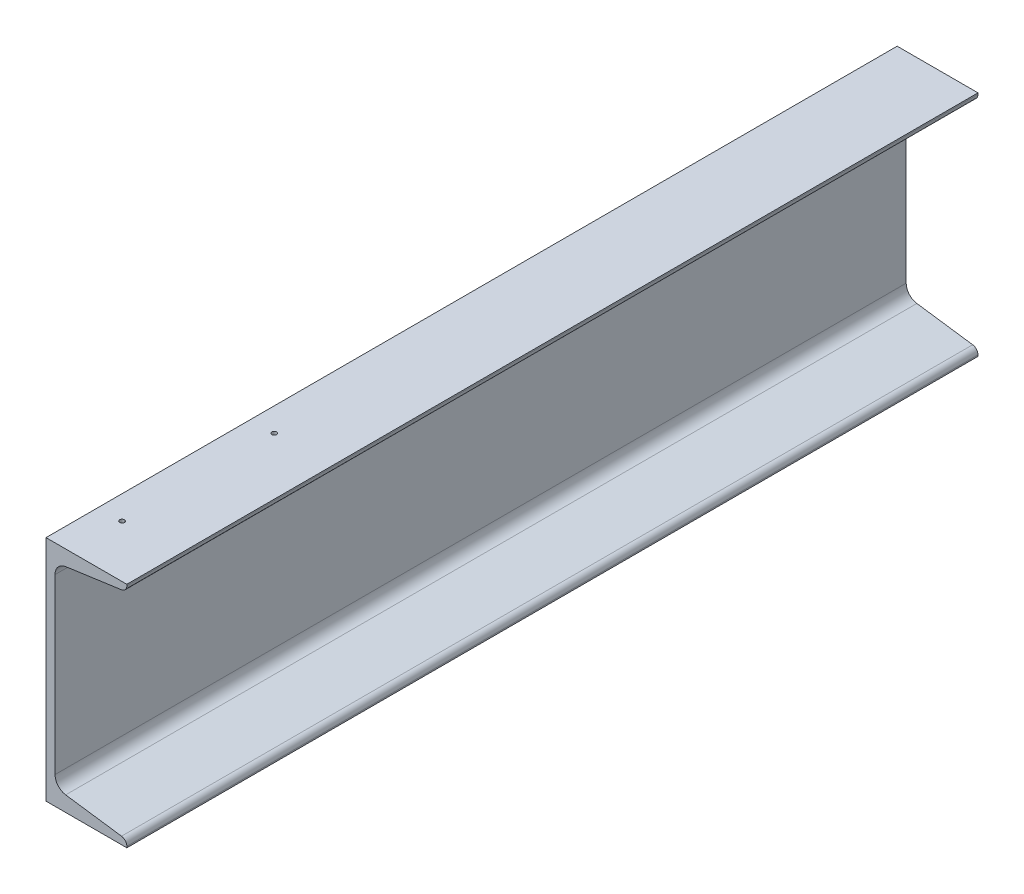
from build123d import *

# Parameters (mm, degrees)
EXTRUDE_1_DEPTH        = 895
HOLE_WIZARD_M8_1_D     = 6.8
HOLE_WIZARD_M8_1_DEPTH = 19.75
HOLE_WIZARD_M8_1_TIP   = 2.042926105
HOLE_WIZARD_M6_1_D     = 5
HOLE_WIZARD_M6_1_DEPTH = 15
HOLE_WIZARD_M6_1_TIP   = 1.502151548


with BuildPart() as part:
    # 草图1 → 凸台-拉伸1 (new body)
    with BuildSketch(Plane.XY):
        with BuildLine():
            Line((0, 0), (-85, 0))
            Line((-85, 0), (-85, -240))
            Line((-85, -240), (0, -240))
            Line((0, -240), (0, -238.623349271))
            ThreePointArc((0, -238.623349271), (-1.594387729, -234.358965582), (-5.595374844, -232.186606824))
            Line((-5.595374844, -232.186606824), (-64.309250312, -223.934909757))
            ThreePointArc((-64.309250312, -223.934909757), (-72.311224543, -219.59019224), (-75.5, -211.061424863))
            Line((-75.5, -211.061424863), (-75.5, -28.938575137))
            ThreePointArc((-75.5, -28.938575137), (-72.311224543, -20.40980776), (-64.309250312, -16.065090243))
            Line((-64.309250312, -16.065090243), (-5.595374844, -7.813393176))
            ThreePointArc((-5.595374844, -7.813393176), (-1.594387729, -5.641034418), (0, -1.376650729))
            Line((0, -1.376650729), (0, 0))
        make_face()
    extrude(amount=EXTRUDE_1_DEPTH)

    # M8 螺纹孔1
    with Locations(Plane.ZY.offset(85)):
        with Locations((630, -50), (710, -50)):
            Hole(HOLE_WIZARD_M8_1_D / 2, depth=HOLE_WIZARD_M8_1_DEPTH)
            with Locations((0, 0, -(HOLE_WIZARD_M8_1_DEPTH + HOLE_WIZARD_M8_1_TIP / 2))):  # 118° drill point
                Cone(0, HOLE_WIZARD_M8_1_D / 2, HOLE_WIZARD_M8_1_TIP, mode=Mode.SUBTRACT)

    # M6 螺纹孔1
    with Locations(Plane(origin=(0, 0, 0), x_dir=(1, 0, 0), z_dir=(0, 1, 0))):
        with Locations((-60, -840), (-60, -680)):
            Hole(HOLE_WIZARD_M6_1_D / 2, depth=HOLE_WIZARD_M6_1_DEPTH)
            with Locations((0, 0, -(HOLE_WIZARD_M6_1_DEPTH + HOLE_WIZARD_M6_1_TIP / 2))):  # 118° drill point
                Cone(0, HOLE_WIZARD_M6_1_D / 2, HOLE_WIZARD_M6_1_TIP, mode=Mode.SUBTRACT)


solid = part.part
